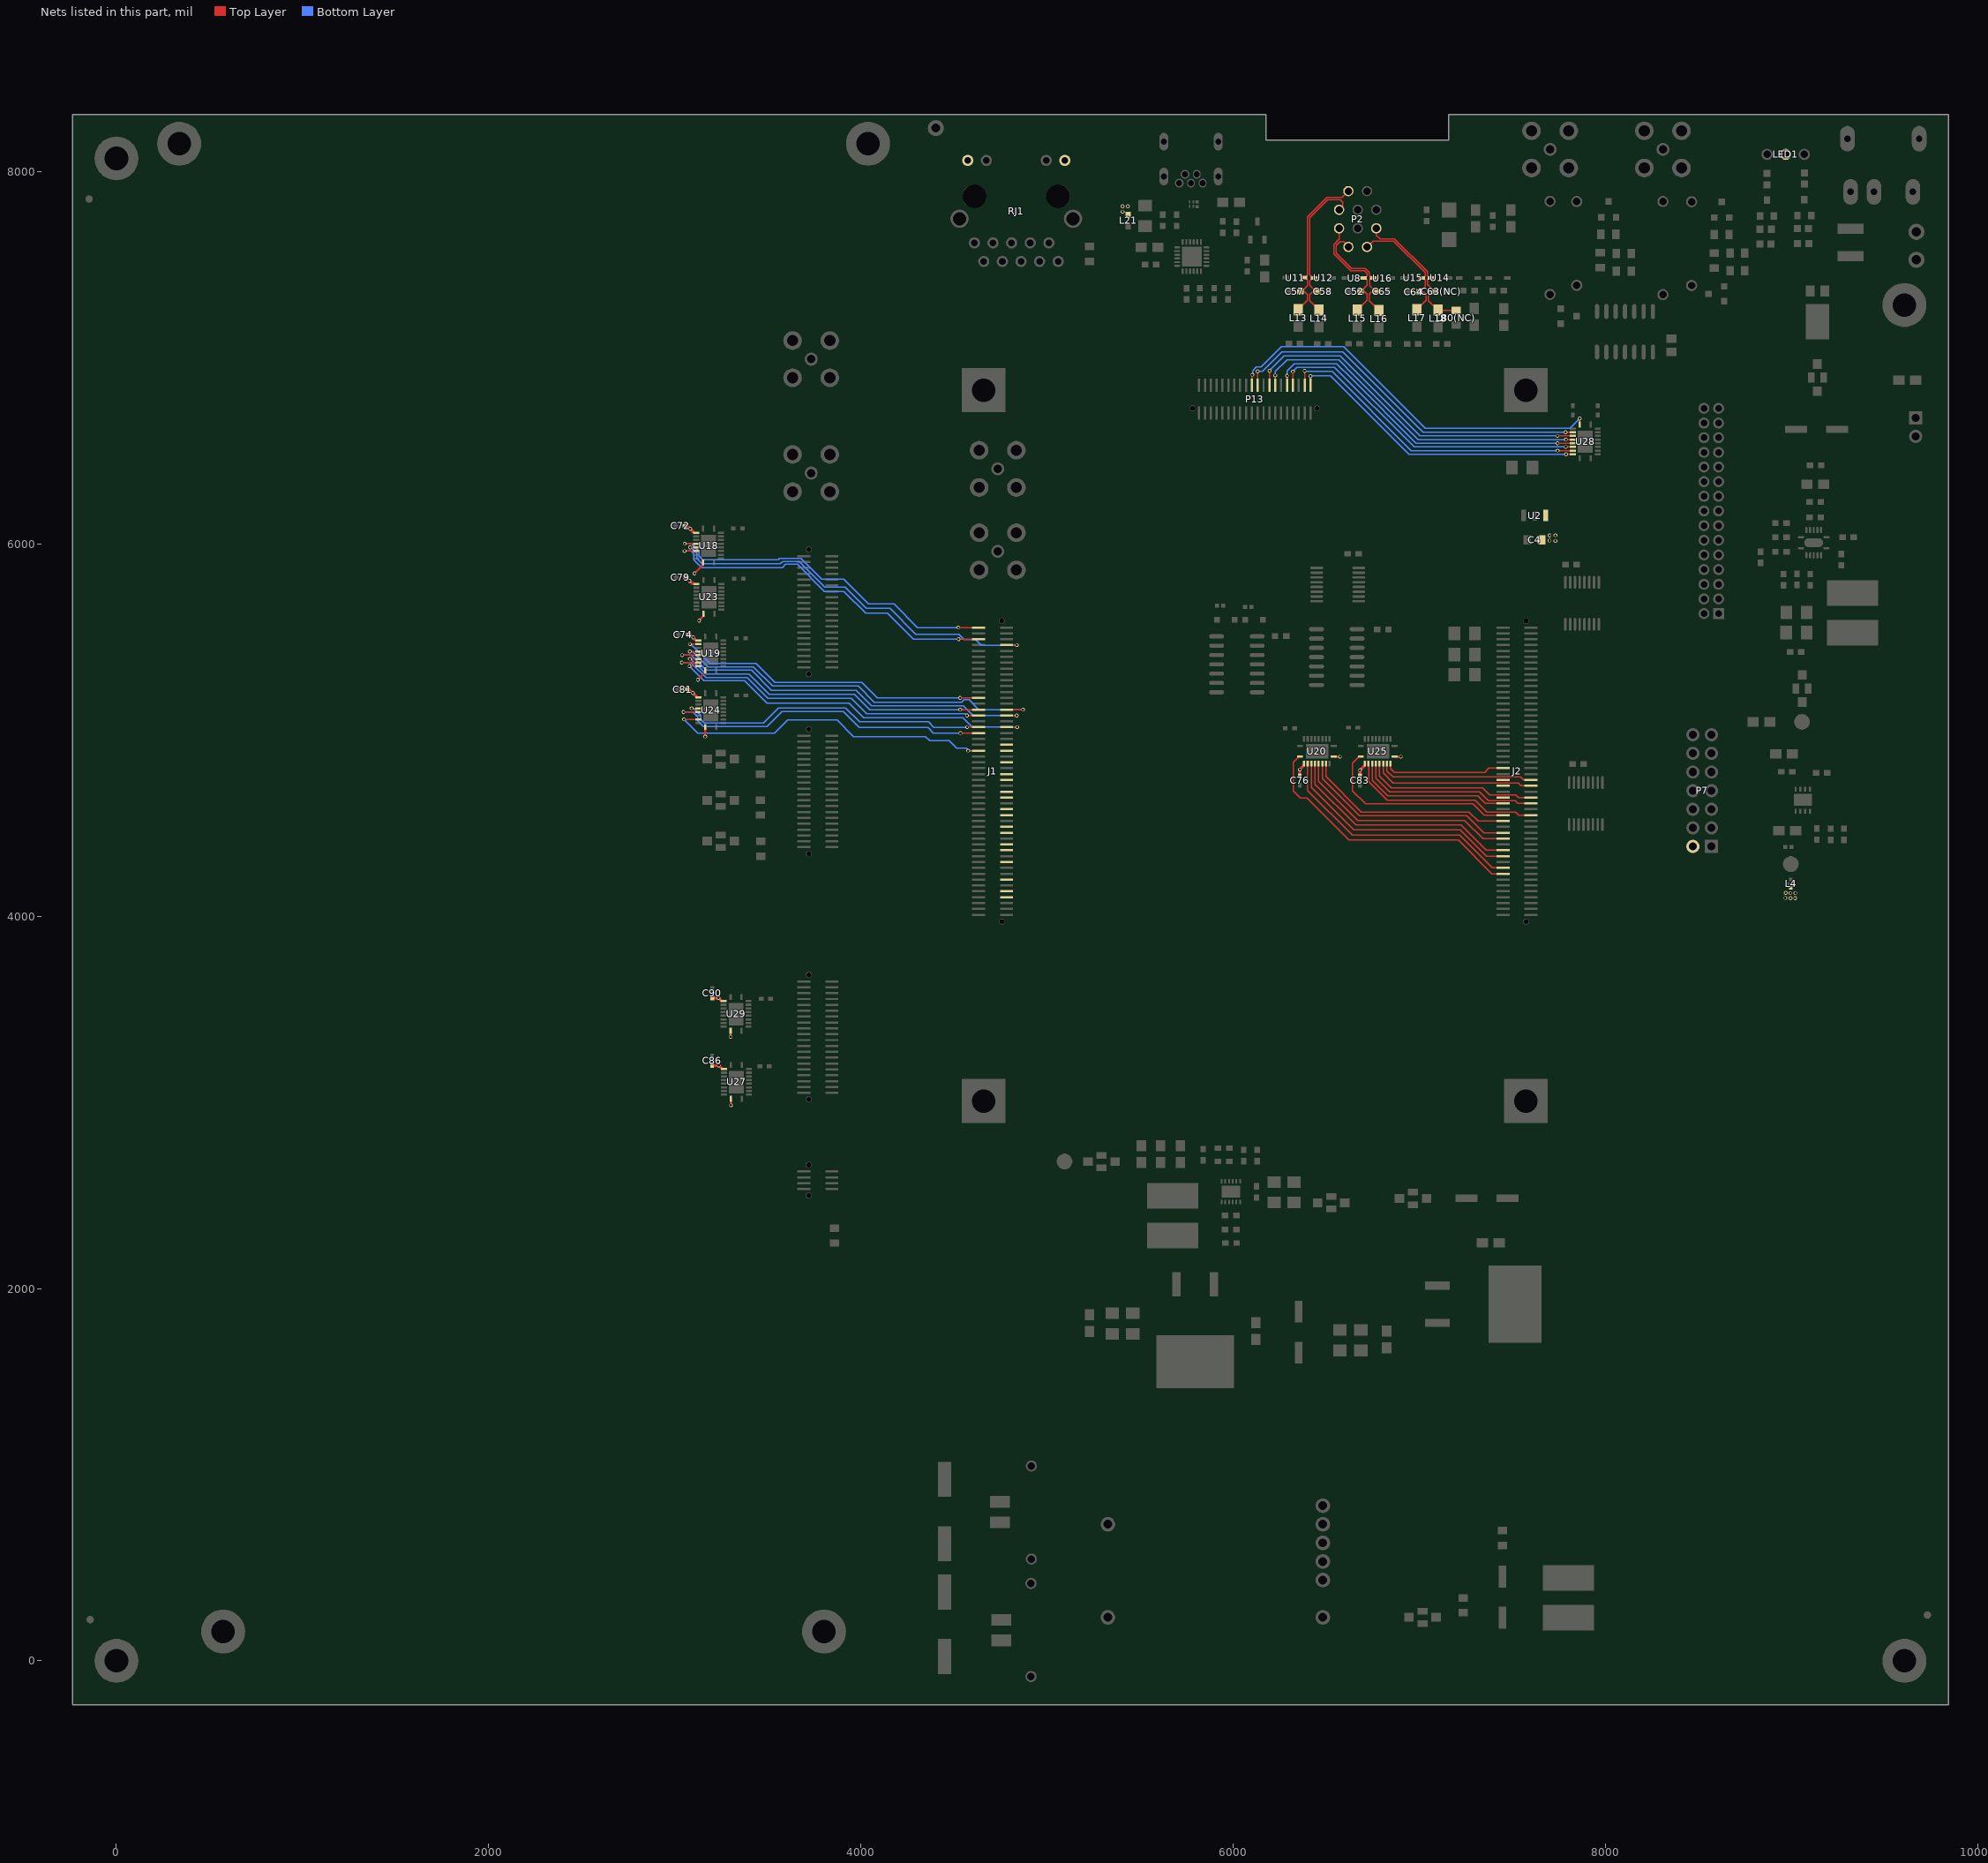
[diagram p0: the nets of this part, all layers, seen from the top]
# Altium PCB MISC82191.PcbDoc (part 3 of 9)
Units mil, origin at the board's own origin, x right, y up, seen from the top; angles counter-clockwise.
Board outline 10078.74 x 8543.31 mil, 4 copper layers (Top Layer, GND, POWER, Bottom Layer); 238 components, 299 nets, 1297 pads, 1665 vias.

## Footprints (in the part's own frame and the unit in brackets; to place one, negate y for a bottom-side part, rotate by r counter-clockwise, add the part's x,y. Pads: shape width x height; smd on the part's side, far side on the other; paste and mask are expansions set on the pad) (continued)
SOD-323 [mm]
  rect 0.9x0.5 smd: 1(-1.25,0) 2(1.25,0)
  Top Layer pour cut-out: -0.635,0.635 0.635,0.635 0.635,-0.635 -0.635,-0.635
  silkscreen extent -1.51,-0.62 1.5,0.62
SOT23 [mil]
  rect 35x40 smd: 1(0,0) 2(75,0) 3(37.5,85)
  silkscreen extent -20,19 93,69
SOT-23 [mil]
  rect 35x35 smd: 1(0,0) 2(80,0) 3(40,85)
  silkscreen extent -21,19 96,69
SOT-23-3_L2.9-W1.6-P1.90-LS2.8-BR [mm]
  rect 1.07x0.6 smd: 1(0,0) 2(0,1.9) 3(-2.47,0.95)
  silkscreen extent -2.11,-0.59 -0.36,2.49
SOT-89-3_L4.5-W2.5-P1.50-LS4.2-BR [mm]
  rect 1.575x0.672 smd: 1(0,0) 3(0,3)
  rect 1.27x0.508 smd: 2(0.034,1.507)
  Top Layer region: -3.64,2.45 -1.785,2.45 -1.741,2.449 -1.696,2.446 -1.652,2.44 -1.608,2.433 -1.565,2.424 -1.522,2.412 -1.479,2.399 -1.437,2.384 -1.396,2.366 -1.356,2.347 -1.317,2.326 -1.279,2.303 -1.241,2.279 -1.206,2.252 -1.171,2.224 -1.138,2.195 -1.106,2.164 -1.075,2.131 -1.047,2.097 -1.019,2.062 -0.994,2.025 -0.97,1.987 -0.948,1.949 -0.928,1.909 -0.91,1.83 0.788,1.83 0.788,1.17 -0.91,1.17 -0.928,1.09 -0.948,1.051 -0.97,1.012 -0.994,0.974 -1.019,0.938 -1.047,0.902 -1.075,0.868 -1.106,0.836 -1.138,0.805 -1.171,0.775 -1.206,0.747 -1.241,0.721 -1.279,0.696 -1.317,0.673 -1.356,0.652 -1.396,0.633 -1.437,0.616 -1.479,0.6 -1.522,0.587 -1.565,0.576 -1.608,0.566 -1.652,0.559 -1.696,0.554 -1.741,0.551 -1.785,0.55 -3.64,0.55 -3.684,0.551 -3.728,0.554 -3.773,0.559 -3.817,0.566 -3.86,0.576 -3.903,0.587 -3.946,0.6 -3.988,0.616 -4.029,0.633 -4.069,0.652 -4.108,0.673 -4.146,0.696 -4.183,0.721 -4.219,0.747 -4.254,0.775 -4.287,0.805 -4.319,0.836 -4.349,0.868 -4.378,0.902 -4.405,0.938 -4.431,0.974 -4.455,1.012 -4.477,1.051 -4.497,1.09 -4.515,1.131 -4.531,1.172 -4.546,1.215 -4.558,1.257 -4.568,1.301 -4.577,1.344 -4.583,1.389 -4.587,1.433 -4.589,1.477 -4.589,1.522 -4.587,1.566 -4.583,1.611 -4.577,1.655 -4.568,1.699 -4.558,1.742 -4.546,1.785 -4.531,1.827 -4.515,1.868 -4.497,1.909 -4.477,1.949 -4.455,1.987 -4.431,2.025 -4.405,2.062 -4.378,2.097 -4.349,2.131 -4.319,2.164 -4.287,2.195 -4.254,2.224 -4.219,2.252 -4.183,2.279 -4.146,2.303 -4.108,2.326 -4.069,2.347 -4.029,2.366 -3.988,2.384 -3.946,2.399 -3.903,2.412 -3.86,2.424 -3.817,2.433 -3.773,2.44 -3.728,2.446 -3.684,2.449
  silkscreen extent -3.31,-0.83 -0.65,3.83
TDFN-12_L3.0-W3.0-P0.50-BL-EP [mm]
  rect 0.25x0.6 smd: 1(0,0) 2(0.5,0) 3(1,0) 4(1.5,0) 5(2,0) 6(2.5,0) 7(2.5,2.8) 8(2,2.8) 9(1.5,2.8) 10(1,2.8) 11(0.5,2.8) 12(0,2.8)
  rect 2.5x1.6 smd: 13(1.25,1.4)
  silkscreen extent -0.63,-0.72 2.92,2.9
TO-263-2_L10.0-W9.1-P5.08-LS15.2-TL [mil]
  rect 132.23x44.65 smd: 1(0,0) 3(0,-200)
  rect 282.7x416 smd: 4(416.21,-100)
  silkscreen extent -48,-303 269,103
TP1 [mil]
  round 85 smd: 1(0,0)
TSSOP-16_L5.0-W4.4-P0.65-LS6.4-BL [mm]
  oval 0.343x1.731 smd: 1(0,0) 2(0.65,0) 3(1.3,0) 4(1.95,0) 5(2.6,0) 6(3.25,0) 7(3.9,0) 8(4.55,0) 9(4.55,5.732) 10(3.9,5.732) 11(3.25,5.732) 12(2.6,5.732) 13(1.95,5.732) 14(1.3,5.732) 15(0.65,5.732) 16(0,5.732)
  silkscreen extent -0.77,-0.15 4.85,4.64
VQFN-14_L3.5-W3.5-P0.50-BL-EP_TPS54622RHLT [mm]
  oval 0.85x0.28 smd: 1(0,0) 7(3.45,-0.003) 8(3.45,1.5) 14(0,1.5)
  oval 0.28x0.85 smd: 2(0.725,-0.975) 3(1.225,-0.975) 4(1.725,-0.975) 5(2.225,-0.975) 6(2.725,-0.975) 9(2.725,2.475) 10(2.225,2.475) 11(1.725,2.475) 12(1.225,2.475) 13(0.725,2.475)
  oval 2.592x1.219 smd: 15(1.725,0.75)
  Top Layer region: 0.709,-0.266 0.709,0.35 -0.435,0.35 -0.435,0.59 0.285,0.59 0.285,0.91 -0.435,0.91 -0.435,1.15 0.709,1.15 0.709,1.766 2.741,1.766 2.741,1.15 3.885,1.15 3.885,0.91 3.165,0.91 3.165,0.59 3.885,0.59 3.885,0.35 2.741,0.35 2.741,-0.266 0.709,-0.266
  silkscreen extent -0.8,-1.15 3.62,2.65
板对板座2*50 [mm]
  round 0.8 hole 0.68: 0(-40.129,0.638) 0(0.9,0.65)
  rect 0.3x1.8 smd: A1(0,0) A2(-0.8,0) A3(-1.6,0) A4(-2.4,0) A5(-3.2,0) A6(-4,0) A7(-4.8,0) A8(-5.6,0) A9(-6.4,0) A10(-7.2,0) A11(-8,0) A12(-8.8,0) A13(-9.6,0) A14(-10.4,0) A15(-11.2,0) A16(-12,0) A17(-12.8,0) A18(-13.6,0) A19(-14.4,0) A20(-15.2,0) A21(-15.999,0) A22(-16.799,0) A23(-17.599,0) A24(-18.399,0) A25(-19.199,0) A26(-19.999,0) A27(-20.799,0) A28(-21.599,0) A29(-22.399,0) A30(-23.199,0) A31(-23.999,0) A32(-24.799,0) A33(-25.599,0) A34(-26.399,0) A35(-27.199,0) A36(-27.999,0) A37(-28.799,0) A38(-29.599,0) A39(-30.399,0) A40(-31.199,0) A41(-31.999,0) A42(-32.799,0) A43(-33.599,0) A44(-34.399,0) A45(-35.199,0) A46(-35.999,0) A47(-36.799,0) A48(-37.599,0) A49(-38.399,0) A50(-39.199,0) B1(0,3.8) B2(-0.8,3.8) B3(-1.6,3.8) B4(-2.4,3.8) B5(-3.2,3.8) B6(-4,3.8) B7(-4.8,3.8) B8(-5.6,3.8) B9(-6.4,3.8) B10(-7.2,3.8) B11(-8,3.8) B12(-8.8,3.8) B13(-9.6,3.8) B14(-10.4,3.8) B15(-11.2,3.8) B16(-12,3.8) B17(-12.8,3.8) B18(-13.6,3.8) B19(-14.4,3.8) B20(-15.2,3.8) B21(-15.999,3.8) B22(-16.799,3.8) B23(-17.599,3.8) B24(-18.399,3.8) B25(-19.199,3.8) B26(-19.999,3.8) B27(-20.799,3.8) B28(-21.599,3.8) B29(-22.399,3.8) B30(-23.199,3.8) B31(-23.999,3.8) B32(-24.799,3.8) B33(-25.599,3.8) B34(-26.399,3.8) B35(-27.199,3.8) B36(-27.999,3.8) B37(-28.799,3.8) B38(-29.599,3.8) B39(-30.399,3.8) B40(-31.199,3.8) B41(-31.999,3.8) B42(-32.799,3.8) B43(-33.599,3.8) B44(-34.399,3.8) B45(-35.199,3.8) B46(-35.999,3.8) B47(-36.799,3.8) B48(-37.599,3.8) B49(-38.399,3.8) B50(-39.199,3.8)
  silkscreen extent -41.33,-0.41 1.6,4

## Part data
C3 C4 C104 C105 C109 C110: library part CAPACITOR, "Generic Capacitor"
C5 C12 C13 C14: library part C1206
C6 C7: library part C0402
C8 C9 C10 C11 C16 C17 C18 C19 C20 C21 C24 C25 C26 C27 C35 C36 C37 C39 C40 C41 C42 C43 C44 C45 C46 C47 C48 C49 C50 C51 C91 C92 C95 C96 C97 C102 C112 C115 C116 C117 C704 C706: library part CAP, "Capacitor"
C15 C23 C38 C100: library part CAPACITOR_1, "Capacitor"
C52 C53 C54 C55 C56 C57 C58 C59 C60 C61 C62 C63(NC) C64 C65 C66 C67 C68（NC） C69 C70 C501 C502: library part CAP, "CC-50V-106-±10%-[1206]"
C71 C72 C73 C74 C75 C76 C77 C78 C79 C80 C81 C82 C83 C85 C86 C87 C88 C89 C90 C98 C103: library part CAP
C99 C101 C111: library part CAPACITOR, "Capacitor"
C106 C107 C108: library part CAP1
CN1: library part ZX-XH2.54-2PZZ
D2 D3: library part D
D4 D5: library part D1, "Diode"
F1 F2 F3: library part "Fuse 1", "Fuse"
FB1: library part "Ferrite Bead", "Generic Ferrite Bead"
IC1: "3PEAK"
J4: library part Micro_USB2_0.0_DIP1
L2 L10 L20: library part L
L4: library part YFF31HC2A105MT000N
L11 L12 L13 L14 L15 L16 L17 L18 L19 L21 L80(NC): library part L, "BLM18KG601SN-[0603]/Murata"
LED1: library part LED_2
P2: "Header, 10-Pin"
P4 P6 P9 P13: "Header, 20-Pin, Dual row"
P7: "Header, 7-Pin, Dual row"
P8 P10 P50 P51 P52 P53: library part JA1
P11: "Header, 4-Pin, Dual row"
Q1 Q2: library part NPN, "NPN Transistor"
Q3 Q4: library part PNP, "PNP Transistor"
R1 R3 R6: library part R0603
R2 R4 R5 R7 R8 R9 R12 R13 R14 R19 R20 R25 R26 R27 R28 R35 R36 R37 R38 R39 R40 R41 R42 R43 R44 R45 R46 R47 R48 RZ1 RZ2: library part RES1
R23 R34: library part RES
TP1 TP2 TP4: library part TEST_2
U2: library part AMS1117S-3.3
U3: library part TPS54620RGYR
U5 U6: library part L7809CD2T-TR
U7: library part TPS63710DRRR
U8 U9 U10 U11 U12 U14 U15 U16: library part "SMAJ18CA 18V", "BV05C-[SOD-323]/Bencent"
U13: library part "SMAJ18CA 18V"
U17 U21 U22: library part AM26LV32EIPWR
U26 U501 U707: library part 74HC14D,653
U34: library part XC6206P332MR

## Free pads (board coordinates)
  round 236.22 hole 125.98: 0(0,8070.87) 0(573.48,157.48) 0(3801.83,157.48) 1(9606.3,0) 2(4038.05,8149.61) 2(9606.3,7283.46) 3(0,0) 3(337.26,8149.61)
  rect 236.22x236.22 hole 125.98: 0(4659.19,3007.09) 0(4659.19,6825.99) 0(7572.57,3007.09) 0(7572.57,6825.99)
  round 86.61 hole 47.24: 1(4402.78,8233.78)
  round 39.37 smd mask+39.37: MARK(-147.22,7852.41) MARK(-141.22,221.41) MARK(9729.78,246.41)
  round 39.37 smd far side mask+39.37: MARK(-147.22,7852.41) MARK(-141.22,221.41) MARK(9729.78,246.41)

## Via types
v1: diameter 20, hole 12, Top Layer to Bottom Layer, 1664 vias
v2: diameter 40, hole 20, Top Layer to Bottom Layer, 1 vias

## Nets (pads, with @x,y where several pads share a name; then routed paths per layer and width w, separated by ;. In a path a pad name is that pad's centre, name@x,y a point inside that pad or via, vN(x,y) a via of type N, cw(c..) or ccw(c..) an arc to the next point about the centre after c; other vN are vias at no path point)
1_A_N: C58.1 L14.2 P2.6 U12.2 | length 837.4
  Top Layer w6: U12.2@6426.78,7430.16 6410.78,7414.16 6410.78,7389.16 C58.1@6438.78,7361.16 ; U12.2@6434.57,7429.16 6427.78,7429.16 6411.78,7445.16 6411.78,7752.19 6508.75,7849.16 6573.78,7849.16 6588.78,7834.16 6588.78,7815.16 P2.6@6573.78,7800.16 ; C58.1@6450.78,7357.16 6429.78,7357.16 6411.28,7338.66 6411.28,7305.66 L14.2@6460.78,7256.16
1_A_P: C57.1 L13.2 P2.5 U11.2 | length 837.6
  Top Layer w6: L13.2@6349.78,7258.16 6399.28,7307.66 6399.28,7338.66 6381.78,7356.16 C57.1@6360.78,7356.16 ; C57.1@6371.78,7361.16 6398.78,7388.16 6398.78,7417.16 U11.2@6391.78,7424.16 ; U11.2@6380.99,7430.16 6386.78,7430.16 6399.78,7443.16 6399.78,7757.16 6503.78,7861.16 6582.78,7861.16 P2.5@6617.78,7896.16
1V8IO1: J1.A21
1V8IO2: J1.A22
1V8IO3: J1.A24
1V8IO4: J1.A27
1V8IO5: J1.A26
1V8IO6: J1.A29
1V8IO7: J1.A30
1V8IO8: J1.A32
1V8IO9: J1.A33
1V8IO10: J1.A35
1V8IO11: J1.A36
1V8IO12: J1.A38
1V8IO13: J1.A39
1V8IO14: J1.A41
1V8IO16: J1.A44
1V8IO17: J1.A46
1V8IO18: J1.A47
1V8IO19: P13.20 U28.1 | length 2116.3
  Top Layer w6: P13.20@6100.13,6852.42 v1@6100.13,6904.51 ; U28.1@7861.78,6641.16 v1(7861.78,6673.16)
  Bottom Layer w6: v1@6104.78,6912.16 6104.78,6930.16 6124.78,6950.16 6149.78,6950.16 6259.78,7060.16 6593.78,7060.16 7032.78,6621.16 7809.78,6621.16 v1(7861.78,6673.16)
  other v1: 6103.78,6909.16
1V8IO20: P13.22 U28.3 | length 1989.2
  Top Layer w6: P13.22@6131.63,6852.42 v1(6131.63,6927.01) ; v1(7786.12,6599.82) U28.3@7824.38,6599.82
  Bottom Layer w6: v1@6134.78,6928.16 6156.78,6928.16 6260.78,7032.16 6587.78,7032.16 6694.78,6925.16 ; 6692.78,6927.16 6694.78,6925.16 ; v1(7786.12,6599.82) 7020.12,6599.82 6694.78,6925.16
1V8IO21: P13.26 U28.4 | length 1918.6
  Top Layer w6: P13.26@6194.62,6852.42 v1(6194.62,6930) ; v1(7741.76,6580.13) U28.4@7824.38,6580.13
  Bottom Layer w6: v1@6193.78,6930.16 6272.78,7009.16 6574.78,7009.16 7003.8,6580.13 v1(7741.76,6580.13)
1V8IO22: P13.28 U28.5 | length 1875.7
  Top Layer w6: P13.28@6226.12,6852.42 v1(6226.12,6904.82) ; v1(7787.07,6560.45) U28.5@7824.38,6560.45
  Bottom Layer w6: v1@6226.78,6906.16 6226.78,6926.16 6288.78,6988.16 6331.78,6988.16 6566.78,6988.16 6653.78,6901.16 ; 6651.78,6903.16 6653.78,6901.16 ; v1(7787.07,6560.45) 6994.49,6560.45 6653.78,6901.16
1V8IO23: P13.32 U28.6 | length 1805
  Top Layer w6: P13.32@6289.11,6852.42 v1(6289.11,6903.83) ; v1(7742.39,6540.76) U28.6@7824.38,6540.76
  Bottom Layer w6: v1@6288.78,6907.16 6288.78,6929.16 6327.78,6968.16 6357.78,6968.16 6555.78,6968.16 6637.78,6886.16 ; 6635.78,6888.16 6637.78,6886.16 ; v1(7742.39,6540.76) 6983.17,6540.76 6637.78,6886.16
1V8IO24: P13.34 U28.7 | length 1756.6
  Top Layer w6: P13.34@6320.61,6852.42 v1(6320.61,6925.33) ; v1(7786.86,6521.08) U28.7@7824.38,6521.08
  Bottom Layer w6: v1@6324.78,6931.16 6341.96,6948.34 6544.6,6948.34 6971.86,6521.08 v1(7786.86,6521.08)
1V8IO25: P13.38 U28.8 | length 1694.5
  Top Layer w6: P13.38@6383.6,6852.42 v1(6383.6,6929.34) ; v1(7743.02,6501.39) U28.8@7824.38,6501.39
  Bottom Layer w6: v1@6382.78,6926.16 6530.78,6926.16 6955.54,6501.39 v1(7743.02,6501.39)
1V8IO26: P13.40 U28.9 | length 1633.2
  Top Layer w6: P13.40@6415.09,6852.42 v1(6415.09,6901.47) ; v1(7788.33,6481.71) U28.9@7824.38,6481.71
  Bottom Layer w6: v1@6419.78,6903.16 6522.78,6903.16 6579.28,6846.66 ; 6575.78,6850.16 6579.28,6846.66 ; v1(7788.33,6481.71) 6944.23,6481.71 6579.28,6846.66
2_A_N: C65.2 L16.2 P2.8 U16.1 | length 626.8
  Top Layer w6: P2.8@6618.78,7595.16 6618.78,7599.16 6592.78,7625.16 6574.78,7625.16 6552.78,7603.16 6552.78,7563.13 6636.75,7479.16 6708.78,7479.16 6730.78,7457.16 6730.78,7443.16 6745.78,7428.16 U16.1@6752.57,7428.16 ; 6731.78,7333.16 6731.78,7331.16 ; U16.1@6743.78,7428.16 6732.78,7417.16 6732.78,7386.16 C65.2@6755.78,7363.16 ; C65.2@6768.78,7355.16 6744.78,7355.16 6731.78,7342.16 6731.78,7331.16 ; L16.2@6783.78,7254.16 6731.78,7306.16 6731.78,7331.16
2_A_P: C52.1 L15.2 P2.7 U8.2 | length 626.1
  Top Layer w6: P2.7@6569.78,7687.16 6569.78,7637.13 6540.78,7608.13 6540.78,7558.16 6631.78,7467.16 6703.81,7467.16 6718.78,7452.19 6718.78,7439.16 6707.78,7428.16 U8.2@6699.99,7428.16 ; L15.2@6667.78,7256.16 6719.78,7308.16 6719.78,7330.16 ; C52.1@6683.78,7356.16 6704.78,7356.16 6719.78,7341.16 6719.78,7330.16 ; C52.1@6696.78,7367.16 6719.78,7390.16 6719.78,7417.16 U8.2@6708.78,7428.16 ; 6719.78,7333.16 6719.78,7330.16
3_A_N: C63(NC).2 L18.2 L80(NC).2 P2.2 U14.1 | length 760.2
  Top Layer w6: P2.2@6769.78,7687.16 6769.78,7658.16 6789.78,7638.16 6866.78,7638.16 7042.78,7462.16 7042.78,7442.16 7055.78,7429.16 U14.1@7061.57,7429.16 ; 7048.78,7335.16 7048.78,7334.16 ; U14.1@7053.78,7429.16 7043.78,7419.16 7043.78,7393.16 7075.78,7361.16 ; 7086.78,7355.16 7062.78,7355.16 7048.78,7341.16 7048.78,7334.16 ; L18.2@7099.78,7256.16 7048.78,7307.16 7048.78,7334.16 ; L18.2@7100.85,7255.09 7197.4,7255.09
3_A_P: C64.2 L17.2 P2.1 U15.1 | length 662.5
  Top Layer w6: P2.1@6725.78,7599.16 6752.78,7626.16 6861.81,7626.16 7030.78,7457.19 7030.78,7439.16 7020.78,7429.16 U15.1@7013.99,7429.16 7019.78,7429.16 7031.78,7417.16 7031.78,7383.16 C64.2@7010.78,7362.16 ; L17.2@6985.78,7258.16 7036.78,7309.16 7036.78,7330.16 ; C64.2@6999.78,7354.16 7022.78,7354.16 7036.78,7340.16 7036.78,7330.16 ; 7036.78,7335.16 7036.78,7330.16
3V3: C4.2 C72.2 C74.2 C76.2 C79.2 C81.2 C83.2 C86.2 C90.2 L4.3 L21.2 LED1.2 P7.2 RJ1.11 RJ1.14 U2.3 U18.2 U18.10 U19.2 U19.10 U20.2 U20.10 U23.2 U23.10 U24.2 U24.10 U25.2 U25.10 U27.2 U27.10 U29.2 U29.10 | length 867.5
  Top Layer w11: v1(3105.78,5841.16) 3151.68,5887.06 U18.10@3151.68,5900.68 ; v1(3123.78,5270.16) 3163.78,5310.16 U19.10@3163.78,5321.68 ; v1(3130.78,5588.16) 3130.78,5590.16 3153.78,5613.16 U23.10@3153.78,5624.68 ; v1(3163.78,4965.16) U24.10@3163.78,5016.68 ; U27.2@3253.28,3180.66 3254.81,3179.13 U27.2@3264.38,3179.13 ; v1(3299.78,3352.16) U29.10@3299.78,3384.68 ; v1(3301.78,2984.16) U27.10@3301.78,3019.68 ; U20.10@6539.91,4856.72 v1(6573.35,4856.72) ; U25.10@6866.91,4856.72 v1(6900.35,4856.72)
  Top Layer w16: C72.2@3054.78,6097.16 3065.78,6097.16 v1@3082.28,6080.66 ; C79.2@3056.78,5820.16 3059.78,5820.16 v1@3079.78,5800.16 ; C81.2@3066.78,5219.16 3076.78,5219.16 v1(3096.78,5199.16) U24.2@3117.78,5178.16 ; C74.2@3069.78,5512.16 3083.78,5512.16 v1@3098.28,5497.66 ; v1(3078.78,5801.16) v1@3079.78,5800.16 ; v1(3082.78,6081.16) v1@3082.28,6080.66 ; v1(3098.78,5498.16) v1@3098.28,5497.66 ; 3099.78,5786.16 3093.78,5786.16 v1@3079.78,5800.16 ; U18.2@3099.78,6063.16 v1@3082.28,6080.66 ; U19.2@3111.78,5484.16 v1@3098.28,5497.66 ; C86.2@3200.78,3199.16 v1@3235.78,3199.16 ; C90.2@3206.78,3561.16 v1@3235.78,3561.16 ; v1(3234.78,3561.16) v1@3235.78,3561.16 ; v1(3235.78,3198.16) v1@3235.78,3199.16 ; U29.2@3249.78,3547.16 v1@3235.78,3561.16 ; U27.2@3253.78,3181.16 v1@3235.78,3199.16 ; C76.2@6357.78,4754.16 v1(6357.78,4788.16) U20.2@6377.78,4808.16 ; C83.2@6680.78,4754.16 v1@6680.78,4784.16 ; v1(6681.78,4785.16) v1@6680.78,4784.16 ; U25.2@6702.78,4806.16 v1@6680.78,4784.16
  other v1: 8994.78,4097.16 9018.78,4097.16 8966.78,4098.16 8993.78,4124.16 9019.78,4124.16 8968.78,4125.16 7730.78,6016.16 7699.78,6018.16 7699.78,6045.16 7730.78,6046.16 5405.78,7784.16 5405.78,7813.16 5433.78,7813.16
3VIO23: J1.B19 U24.6 | length 1790.6
  Top Layer w6: v1(3046.55,5097.39) U24.6@3126.38,5097.39 ; v1(4534.67,4984.05) J1.B19@4632.75,4984.05
  Bottom Layer w6: v1(3046.55,5097.39) 3096.42,5097.39 3123.78,5070.03 3123.78,5049.16 3152.78,5020.16 3495.78,5020.16 3574.78,5099.16 3906.03,5099.16 3991.78,5013.41 4359.53,5013.41 4388.88,4984.05 v1(4534.67,4984.05)
3VIO24: J1.B18 U24.5 | length 1813.8
  Top Layer w6: v1(3089.87,5117.07) U24.5@3126.38,5117.07 ; v1(4570.39,5015.55) J1.B18@4632.75,5015.55
  Bottom Layer w6: v1(3089.87,5117.07) 3100.87,5117.07 3139.78,5078.16 3139.78,5057.16 3159.78,5037.16 3475.78,5037.16 3557.78,5119.16 3918.03,5119.16 3992.89,5044.3 4362.89,5044.3 4392.03,5015.16 4499.78,5015.16 ; 4392.78,5015.16 4499.78,5015.16 ; 4551.39,5015.16 4537.78,5015.16 ; v1@4561.78,5015.16 4537.78,5015.16 ; 4499.78,5015.16 4537.78,5015.16
3VIO25: J1.A18 U19.9 | length 2087
  Top Layer w6: v1(3078.95,5343.33) U19.9@3126.38,5343.33 ; J1.A18@4782.37,5015.55 v1(4839.39,5015.55)
  Bottom Layer w6: v1(3078.95,5343.33) 3157.13,5265.16 3374.78,5265.16 3494.78,5145.16 3935.03,5145.16 4014.03,5066.16 4546.78,5066.16 4596.78,5016.16 4728.78,5016.16 ; 4820.39,5016.16 4728.78,5016.16 ; v1@4833.78,5016.16 4728.78,5016.16 ; v1(4839.39,5015.55) v1@4839.78,5015.16
3VIO26: J1.B22 U24.8 | length 1789.8
  Top Layer w6: v1(3048.92,5058.02) U24.8@3126.38,5058.02 ; v1(4576.21,4889.59) J1.B22@4632.75,4889.59
  Bottom Layer w6: v1(3048.92,5058.02) 3122.78,4984.16 3535.78,4984.16 3606.78,5055.16 3871.03,5055.16 3960.78,4965.41 4345.53,4965.41 4368.78,4942.16 4474.78,4942.16 4514.85,4902.09 4565.85,4902.09 v1@4576.78,4891.16
3VIO27: J1.A4 U18.6 | length 2102.7
  Top Layer w6: v1(3082.01,5981.39) U18.6@3114.28,5981.39 ; J1.A4@4782.37,5456.49 v1(4837.44,5456.49)
  Bottom Layer w6: v1(3082.01,5981.39) 3087.55,5981.39 3117.78,5951.16 3117.78,5921.16 3145.78,5893.16 3566.78,5893.16 3579.78,5906.16 3667.78,5906.16 3806.78,5767.16 3913.78,5767.16 4027.53,5653.41 4155.78,5653.41 4295.23,5513.96 4526.98,5513.96 4554.78,5486.16 4616.78,5486.16 4646.78,5456.16 4801.78,5456.16 ; 4818.44,5456.16 4801.78,5456.16 ; v1@4834.78,5456.16 4801.78,5456.16
3VIO28: J1.B16 U19.8 | length 1810
  Top Layer w6: v1(3036.92,5363.02) U19.8@3126.38,5363.02 ; v1(4570.16,5078.54) J1.B16@4632.75,5078.54
  Bottom Layer w6: v1(3036.92,5363.02) 3086.14,5363.02 3097.95,5351.2 3097.95,5350.98 3167.78,5281.16 3389.78,5281.16 3500.78,5170.16 3949,5170.16 4032,5087.16 4431.78,5087.16 4541.78,5087.16 ; 4551.16,5087.16 4541.78,5087.16 ; v1@4567.78,5079.16 4559.78,5087.16 4541.78,5087.16
3VIO29: J1.B15 U19.7 | length 1735
  Top Layer w6: v1(3080.24,5382.7) U19.7@3126.38,5382.7 ; v1(4533.66,5110.04) J1.B15@4632.75,5110.04
  Bottom Layer w6: v1(3080.24,5382.7) 3086.24,5382.7 3168.78,5300.16 3398.78,5300.16 3506.78,5192.16 3914.78,5192.16 ; 3924.78,5192.16 3914.78,5192.16 ; 4514.66,5109.16 4504.78,5109.16 ; v1@4536.78,5109.16 4504.78,5109.16 ; 3914.78,5192.16 3964.03,5192.16 4047.03,5109.16 4403.78,5109.16 4504.78,5109.16
3VIO30: J1.B1 U18.5 | length 1853.5
  Top Layer w6: v1(3052.87,6001.07) U18.5@3114.28,6001.07 ; v1(4522.95,5550.98) J1.B1@4632.75,5550.98
  Bottom Layer w6: v1(3052.87,6001.07) 3089.19,6001.07 3129.78,5960.48 3129.78,5935.16 3148.78,5916.16 3555.78,5916.16 3560.78,5921.16 3678.78,5921.16 3788.78,5811.16 3906.78,5811.16 4040.53,5677.41 4176.78,5677.41 4303.21,5550.98 v1@4518.95,5550.98 ; v1(4522.95,5550.98) v1@4518.95,5550.98 ; v1@4523.78,5546.16 v1@4518.95,5550.98
3VIO31: J1.B3 U18.7 | length 1875
  Top Layer w6: v1(3052.24,5961.7) U18.7@3114.28,5961.7 ; v1(4524.95,5487.99) J1.B3@4632.75,5487.99
  Bottom Layer w6: v1(3052.24,5961.7) 3087.82,5961.7 3100.78,5948.74 3100.78,5916.16 3143.78,5873.16 3578.78,5873.16 3595.89,5890.27 3657.67,5890.27 3803.78,5744.16 3908.78,5744.16 4025.53,5627.41 4142.78,5627.41 4282.2,5487.99 v1@4524.78,5487.99 ; v1@4524.78,5487.16 v1@4524.78,5487.99 ; v1@4524.78,5490.16 v1@4524.78,5487.99 ; v1(4524.95,5487.99) v1@4524.78,5487.99
3VIO32: J1.A16 U19.6 | length 2077.3
  Top Layer w6: v1(3039.01,5402.39) U19.6@3126.38,5402.39 ; J1.A16@4782.37,5078.54 v1(4837.4,5078.54)
  Bottom Layer w6: v1(3039.01,5402.39) 3088.55,5402.39 3168.78,5322.16 3411.78,5322.16 3519.78,5214.16 3973.03,5214.16 4056.03,5131.16 4550.78,5131.16 4603.4,5078.54 v1(4837.4,5078.54) ; v1@4837.4,5077.16 v1@4839.78,5077.16
3VIO33: J1.A15 U19.5 | length 2196
  Top Layer w6: v1(3080.87,5422.07) U19.5@3126.38,5422.07 ; J1.A15@4782.37,5110.04 v1(4870.9,5110.04)
  Bottom Layer w6: v1(3080.87,5422.07) 3094.87,5422.07 3177.78,5339.16 3422.78,5339.16 3525.78,5236.16 3930.78,5236.16 ; 3940.78,5236.16 3930.78,5236.16 ; 4851.9,5110.16 4728.78,5110.16 ; v1@4869.78,5110.16 4728.78,5110.16 ; 3930.78,5236.16 3985.03,5236.16 4071.03,5150.16 4541.78,5150.16 4554.78,5163.16 4580.78,5163.16 4633.78,5110.16 4728.78,5110.16
3VIO34: J1.B13 U19.3 | length 1715.6
  Top Layer w6: v1(3081.5,5461.44) U19.3@3126.38,5461.44 ; v1(4532.65,5173.03) J1.B13@4632.75,5173.03
  Bottom Layer w6: v1(3081.5,5461.44) 3085.5,5461.44 3189.78,5357.16 3435.78,5357.16 3537.78,5255.16 4005.03,5255.16 4087.16,5173.03 v1(4532.65,5173.03)
3VIO40: J2.B27
3VIO41: J2.B28
3VIO42: J2.B30
3VIO43: J2.B25 U25.9 | length 646.8
  Top Layer w6: U25.9@6845.25,4819.32 6845.25,4794.68 6866.78,4773.16 7350.78,4773.16 7372.72,4795.1 J2.B25@7449.4,4795.1
3VIO44: J2.B31 U25.4 | length 843.1
  Top Layer w6: U25.4@6746.83,4819.32 6746.83,4730.11 6829.78,4647.16 7312.78,4647.16 7353.81,4606.13 J2.B31@7449.4,4606.13
3VIO45: J2.B33 U25.1 | length 1056.7
  Top Layer w6: U25.1@6673.78,4855.16 6641.78,4823.16 6641.78,4673.16 6710.78,4604.16 7287.78,4604.16 7348.8,4543.13 J2.B33@7449.4,4543.13
3VIO46: J2.B34 U20.8 | length 1118.7
  Top Layer w6: U20.8@6498.57,4819.32 6498.57,4750.37 6688.78,4560.16 7266.78,4560.16 7315.3,4511.64 J2.B34@7449.4,4511.64
3VIO47: J2.B36 U20.7 | length 1170.5
  Top Layer w6: U20.7@6478.88,4819.32 6478.88,4740.06 6679.78,4539.16 7255.78,4539.16 7346.29,4448.65 J2.B36@7449.4,4448.65
3VIO48: J2.B37 U20.6 | length 1211.6
  Top Layer w6: U20.6@6459.2,4819.32 6459.2,4725.74 6669.78,4515.16 7243.78,4515.16 7341.79,4417.15 J2.B37@7449.4,4417.15
3VIO49: J2.B39 U20.5 | length 1260.7
  Top Layer w6: U20.5@6439.78,4813.16 6439.78,4709.16 6658.78,4490.16 7223.78,4490.16 7359.78,4354.16 J2.B39@7449.4,4354.16
3VIO50: J2.B40 U20.4 | length 1309.8
  Top Layer w6: U20.4@6419.83,4819.32 6419.83,4692.11 6648.78,4463.16 7219.78,4463.16 7360.28,4322.66 J2.B40@7449.4,4322.66
3VIO51: J2.B42 U20.3 | length 1365.7
  Top Layer w6: U20.3@6400.14,4819.32 6400.14,4674.8 6639.78,4435.16 7215.78,4435.16 7391.27,4259.67 J2.B42@7449.4,4259.67
3VIO52: J2.B43 U20.1 | length 1503.7
  Top Layer w6: U20.1@6350.78,4855.16 6323.78,4828.16 6323.78,4672.16 6360.78,4635.16 6396.78,4635.16 6622.78,4409.16 7208.78,4409.16 7389.76,4228.17 J2.B43@7449.4,4228.17
3VIO53: J2.A27 U25.8 | length 839.4
  Top Layer w6: U25.8@6825.57,4819.32 6825.57,4780.37 6857.78,4748.16 7424.78,4748.16 ; 7417.78,4748.16 7424.78,4748.16 ; J2.A27@7599.01,4732.11 7559.83,4732.11 7543.78,4748.16 7424.78,4748.16
3VIO54: J2.A28 U25.7 | length 871.7
  Top Layer w6: U25.7@6805.88,4819.32 6805.88,4769.06 6859.42,4715.52 7532.42,4715.52 7547.32,4700.61 J2.A28@7599.01,4700.61
3VIO55: J2.A30 U25.6 | length 926.5
  Top Layer w6: U25.6@6786.2,4819.32 6786.2,4753.74 6849.78,4690.16 7339.78,4690.16 7377.41,4652.53 7517.41,4652.53 7532.32,4637.62 J2.A30@7599.01,4637.62
3VIO56: J2.A31 U25.5 | length 966.4
  Top Layer w6: U25.5@6766.51,4819.32 6766.51,4741.43 6838.78,4669.16 7322.78,4669.16 7370.91,4621.03 7515.91,4621.03 7530.81,4606.13 J2.A31@7599.01,4606.13
3VIO57: J2.A33 U25.3 | length 1120.4
  Top Layer w6: U25.3@6727.78,4818.16 6727.78,4722.16 6827.78,4622.16 7300.78,4622.16 7363.74,4559.19 7449.78,4559.19 ; 7370.74,4559.19 7449.78,4559.19 ; J2.A33@7599.01,4543.13 7534.8,4543.13 7518.74,4559.19 7449.78,4559.19